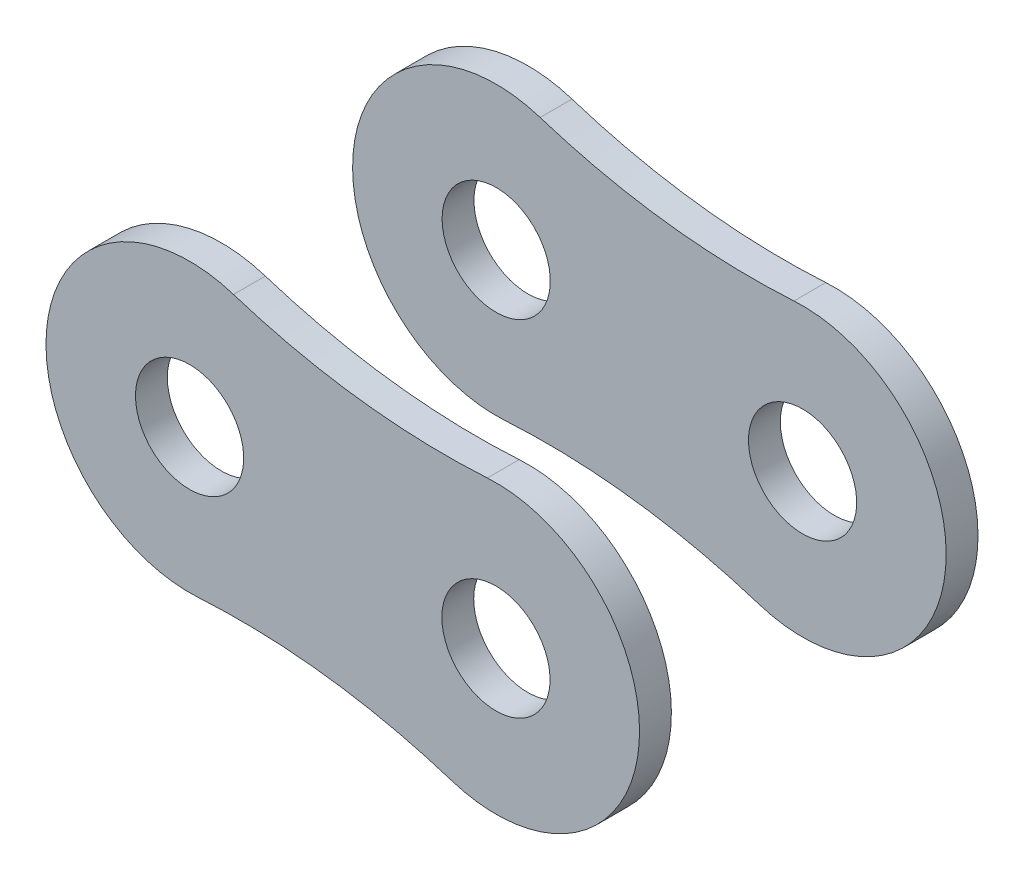
SolidWorks part; units mm, degrees
ref_plane "前视基准面" through (0, 0, 0) normal (0, 0, 1) x (1, 0, 0)
ref_plane "上视基准面" through (0, 0, 0) normal (0, 1, 0) x (1, 0, 0)
ref_plane "右视基准面" through (0, 0, 0) normal (1, 0, 0) x (0, 0, -1)
sketch "草图1" plane through (0, 0, 0) normal (0, 0, 1) x (1, 0, 0)
  line L0 (-6.35, 0) -> (6.35, 0) construction
  line L1 (0, 5.3145) -> (0, -5.3145) construction
  line L2 (6.35, 0) -> (17.65, 0) construction
  line L3 (17.65, 0) -> (25.4, 0) construction
  circle A0 centre (-6.35, 0) radius 5.905
  circle A1 centre (6.35, 0) radius 5.905
  circle A2 centre (0, 33.8474) radius 28.5329
  circle A3 centre (0, -33.8474) radius 28.5329
  circle A4 centre (-6.35, 0) radius 4.255
  circle A5 centre (6.35, 0) radius 4.255
  circle A6 centre (-6.35, 0) radius 2.225
  circle A7 centre (6.35, 0) radius 2.225
  point P16 (37.35, 0)
  point P18 (20.27, 0)
  point P19 (8.35, 0)
sketch "草图2" plane through (0, 0, 0) normal (0, 0, 1) x (1, 0, 0)
  circle A0 centre (6.35, 0) radius 4.255 construction
  circle A1 centre (-6.35, 0) radius 4.255 construction
  circle A2 centre (6.35, 0) radius 4.255
  circle A3 centre (-6.35, 0) radius 4.255
extrude "拉伸1" add sketch "草图2" along normal mid plane 7.75
sketch "草图3" plane through (0, 0, 3.875) normal (0, 0, 1) x (1, 0, 0)
  circle A0 centre (-6.35, 0) radius 5.905 construction
  arc A1 (-5.2612, 5.8037) -> (-5.2612, -5.8037) centre (-6.35, 0) ccw
  circle A2 centre (6.35, 0) radius 5.905 construction
  arc A3 (5.2612, -5.8037) -> (5.2612, 5.8037) centre (6.35, 0) ccw
  circle A4 centre (0, 33.8474) radius 28.5329 construction
  arc A5 (-5.2612, 5.8037) -> (5.2612, 5.8037) centre (0, 33.8474) ccw
  circle A6 centre (0, -33.8474) radius 28.5329 construction
  arc A7 (5.2612, -5.8037) -> (-5.2612, -5.8037) centre (0, -33.8474) ccw
extrude "拉伸2" add sketch "草图3" along normal blind 1.775
sketch "草图5" plane through (0, 0, 0) normal (0, 0, 1) x (1, 0, 0)
  line L0 (6.35, 0) -> (18.9503, -1.5886) construction
  line L1 (-6.35, 0) -> (6.35, 0) construction
  line L2 (-6.35, 0) -> (-775.0628, -48.2675)
  line L4 (0, -101.1307) -> (-770.7315, -117.2475) construction
  line L5 (18.9503, -1.5886) -> (31.2528, -4.7409) construction
  arc A0 (24.8281, -199.3718) -> (-6.35, 0) centre (0, -101.1307) ccw
  arc A1 (-775.0628, -48.2675) -> (-790.2544, -183.5487) centre (-770.7315, -117.2475) ccw
  arc A2 (-790.2544, -183.5487) -> (24.8281, -199.3718) centre (-353.7841, 1298.74) ccw
  dimension "R2" = 202.6597
  dimension "R1" = 138.2317
  dimension "a" = 770.9
  dimension "La" = 770.2266
  dimension "L2" = 299.6078
  dimension "L" = 825
  dimension "L1" = 193.0074
sketch "草图6" plane through (0, 0, 5.65) normal (0, 0, 1) x (1, 0, 0)
  arc A0 (17.144, -7.2106) -> (18.596, 4.3058) centre (18.9503, -1.5886) ccw
  circle A1 centre (6.35, 0) radius 5.905 construction
  arc A2 (8.1562, 5.622) -> (6.7043, -5.8944) centre (6.35, 0) ccw
  arc A3 (8.1562, 5.622) -> (18.596, 4.3058) centre (16.884, 32.7873) ccw
  arc A4 (6.7043, -5.8944) -> (17.144, -7.2106) centre (8.4163, -34.3759) cw
  circle A5 centre (0, 33.8474) radius 28.5329 construction
  circle A6 centre (0, -33.8474) radius 28.5329 construction
  circle A7 centre (6.35, 0) radius 2.225 construction
  circle A8 centre (6.35, 0) radius 2.225
  circle A9 centre (18.9503, -1.5886) radius 2.225
extrude "拉伸4" add sketch "草图6" along normal blind 1.31 separate body
delete or keep bodies "实体-删除1" type delete bodies bodies 103
ref_plane "基准面1" through (0, 0, 0) normal (0, 0, -1) x (-1, 0, 0)
mirror "镜向1" about plane through (0, 0, 0) normal (0, 0, -1) of bodies 123
sketch "草图7" plane through (0, 0, 6.96) normal (0, 0, 1) x (1, 0, 0)
  line L0 (6.35, 0) -> (18.9503, -1.5886)
equation "\"D1@拉伸1\" = \"b1@草图1\""
equation "\"D1@拉伸2\" = (  \"b2@草图1\" - \"D1@拉伸1\" )  / 2"
equation "\"h3@草图1\" = \"h2@草图1\" * 0.9"
equation "\"D1@拉伸4\" = (\"P1@草图1\"-\"b2@草图1\")/2"
